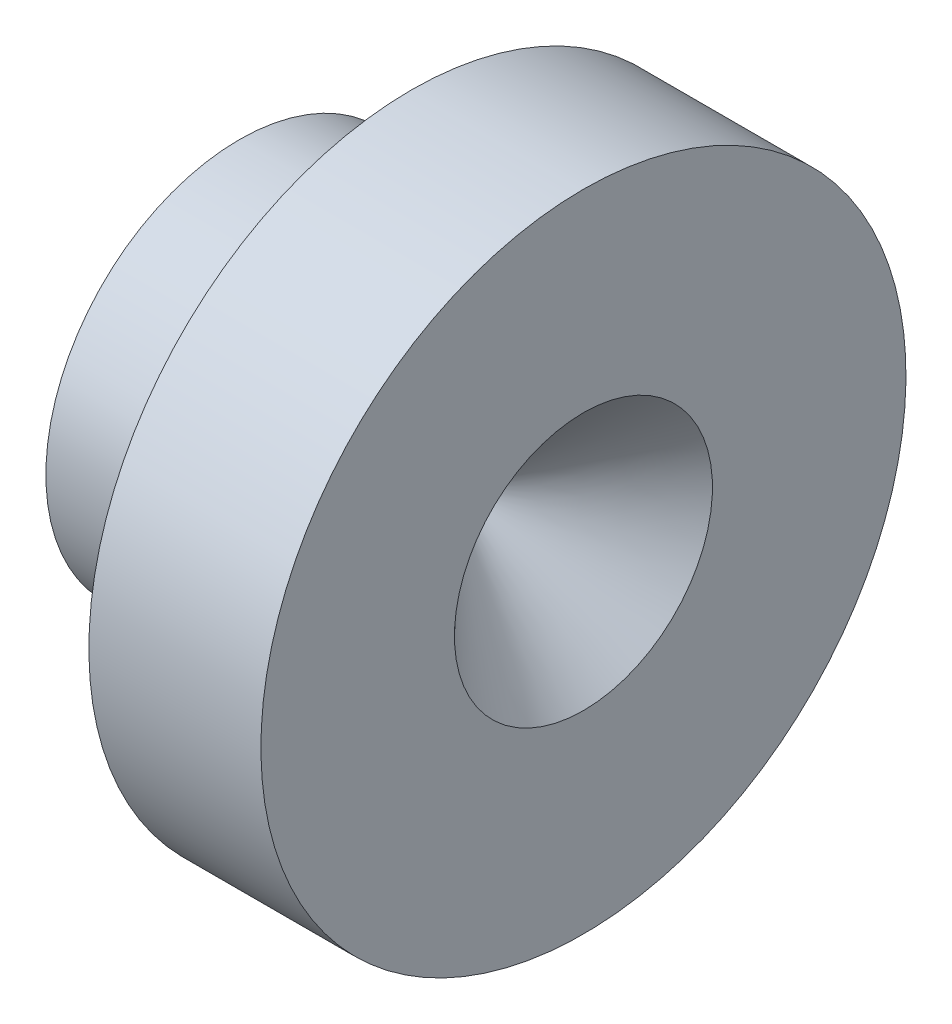
SolidWorks part; units mm, degrees
ref_plane "Front Plane" through (0, 0, 0) normal (0, 0, 1) x (1, 0, 0)
ref_plane "Top Plane" through (0, 0, 0) normal (0, 1, 0) x (1, 0, 0)
ref_plane "Right Plane" through (0, 0, 0) normal (1, 0, 0) x (0, 0, -1)
sketch "Sketch1" plane through (0, 0, 0) normal (0, 0, 1) x (1, 0, 0)
  line L0 (0, 0) -> (0, 4.5)
  line L1 (0, 4.5) -> (4, 4.5)
  line L2 (4, 4.5) -> (4, 7.5)
  line L3 (4, 7.5) -> (8, 7.5)
  line L4 (8, 7.5) -> (8, 3)
  line L5 (8, 0) -> (0, 0)
  line L6 (0, 0.5) -> (5.5, 0.5)
  line L7 (5.5, 0.5) -> (8, 3)
  line L8 (8, 3) -> (8, 0) construction
  dimension "D1" = 4.5
  dimension "D2" = 4
  dimension "D3" = 7.5
  dimension "D4" = 8
  dimension "D5" = 3
  dimension "D6" = 45
  dimension "D7" = 0.5
revolve "Revolve1" add sketch "Sketch1" angle 360 about L5
